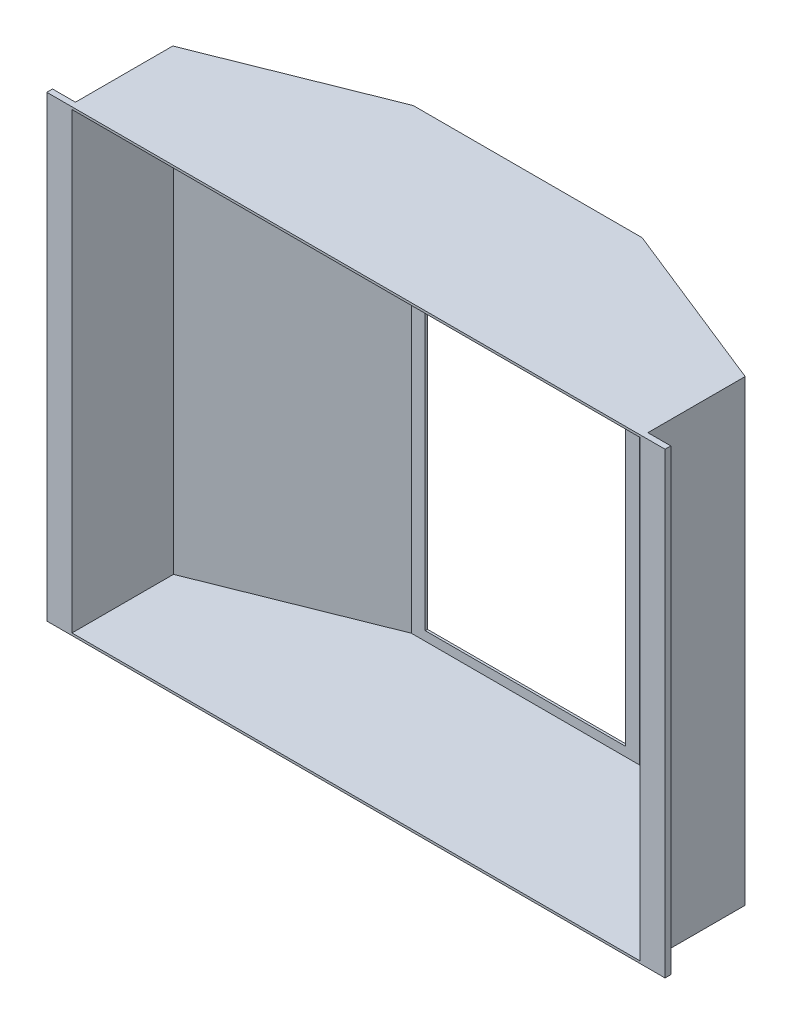
from build123d import *

# Parameters (mm, degrees)
SKETCH_1_W          = 500
SKETCH_1_H          = 400
EXTRUDE_1_DEPTH     = 150
CUT_EXTRUDE_1_DEPTH = 495.974746831
SHELL_1_T           = -2
SKETCH_2_W          = 20
SKETCH_2_H          = 400
EXTRUDE_2_DEPTH     = 5
SKETCH_4_W          = 175
SKETCH_4_H          = 380
CUT_EXTRUDE_2_DEPTH = 368.15664232


with BuildPart() as part:
    # 草图1 → 凸台-拉伸1 (new body)
    with BuildSketch(Plane.XY):
        Rectangle(SKETCH_1_W, SKETCH_1_H)
    extrude(amount=EXTRUDE_1_DEPTH)

    # 草图3 → 切除-拉伸1 (cut, through all)
    with BuildSketch(Plane.XZ.offset(200)):
        Polygon((-100, 0), (-250, 60), (-250, 0), align=None)
        Polygon((250, 60), (100, 0), (250, 0), align=None)
    extrude(amount=-CUT_EXTRUDE_1_DEPTH, mode=Mode.SUBTRACT)

    # 抽壳1
    shell_1_openings = [part.faces().sort_by_distance(p)[0] for p in [
        (0, 0, 150),
    ]]
    offset(amount=SHELL_1_T, openings=shell_1_openings, kind=Kind.INTERSECTION)

    # 草图2 → 凸台-拉伸2 (add)
    with BuildSketch(Plane.XY.offset(150)):
        with Locations((-260, 0)):
            Rectangle(SKETCH_2_W, SKETCH_2_H)
        with Locations((260, 0)):
            Rectangle(SKETCH_2_W, SKETCH_2_H)
    extrude(amount=-EXTRUDE_2_DEPTH)

    # 草图4 → 切除-拉伸2 (cut, through all)
    with BuildSketch(Plane.XY.offset(2)):
        Rectangle(SKETCH_4_W, SKETCH_4_H)
    extrude(amount=-CUT_EXTRUDE_2_DEPTH, mode=Mode.SUBTRACT)


solid = part.part
